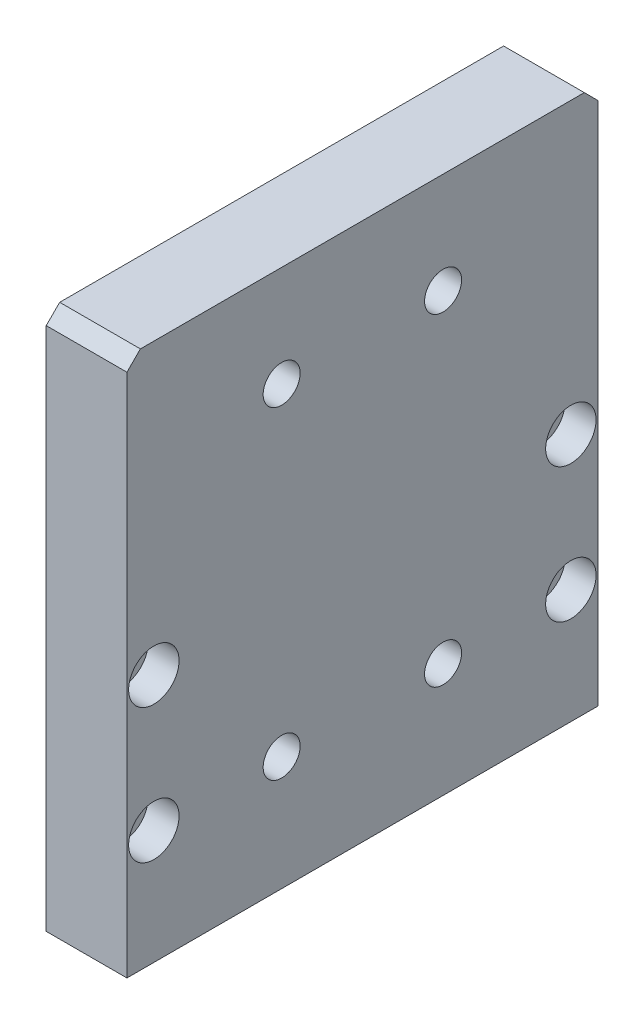
SolidWorks part; units mm, degrees
material "A6061"
ref_plane "前基準面" through (0, 0, 0) normal (0, 0, 1) x (1, 0, 0)
ref_plane "上基準面" through (0, 0, 0) normal (0, 1, 0) x (1, 0, 0)
ref_plane "右基準面" through (0, 0, 0) normal (1, 0, 0) x (0, 0, -1)
sketch "草图1" plane through (0, 0, 0) normal (1, 0, 0) x (0, 0, -1)
  line L1 (-35, 40) -> (35, 40)
  line L2 (-35, 40) -> (-35, -40)
  line L3 (-35, -40) -> (35, -40)
  line L4 (35, 40) -> (35, -40)
  line L5 (-35, 40) -> (35, -40) construction
  line L6 (-35, -40) -> (35, 40) construction
  point P0 (0, 0)
  dimension "D1" = 80
  dimension "D2" = 70
extrude "凸台-拉伸1" add sketch "草图1" along normal blind 12
hole_wizard "M5 六角圆柱头螺钉的柱形沉头孔1" positions "草图2" profile "草图3" counterbore size "M5" standard "GB" end condition through all
sketch "草图2" plane through (0, 0, 0) normal (-1, 0, 0) x (0, 0, 1)
  line L0 (0, 0) -> (0, -50.847) construction
  line L1 (-35, 40) -> (35, 40) construction
  point P0 (-12, 25)
  point P12 (-12, -23)
  point P14 (12, -23)
  point P15 (12, 25)
  dimension "D1" = 24
  dimension "D2" = 48
  dimension "D3" = 15
sketch "草图3" plane through (0, 25, -12) normal (0, 1, 0) x (0, 0, 1)
  line L0 (0, 0) -> (0, 12)
  line L1 (0, 12) -> (2.75, 12)
  line L3 (2.75, 12) -> (2.75, 5.7)
  line L4 (2.75, 5.7) -> (5, 5.7)
  line L5 (5, 5.7) -> (5, 0)
  line L7 (5, 0) -> (0, 0)
  line L11 (0, -6.35) -> (0, 107.95) construction
  dimension "通孔孔直径" = 5.5
  dimension "通孔孔深度" = 12
  dimension "柱形沉头孔直径" = 10
  dimension "柱形沉头孔深度" = 5.7
hole_wizard "M4 六角圆柱头螺钉的柱形沉头孔1" positions "草图4" profile "草图5" counterbore size "M4" standard "GB" end condition through all
sketch "草图4" plane through (12, 0, 0) normal (1, 0, 0) x (0, 0, -1)
  line L0 (0, 0) -> (0, -45.1266) construction
  line L2 (-35, -40) -> (35, -40) construction
  point P0 (-31, -23)
  point P3 (-31, -3)
  point P13 (31, -3)
  point P14 (31, -23)
  dimension "D1" = 62
  dimension "D2" = 20
  dimension "D3" = 17
sketch "草图5" plane through (12, -23, 31) normal (0, 1, 0) x (0, 0, -1)
  line L0 (0, 0) -> (0, 12)
  line L1 (0, 12) -> (2.25, 12)
  line L3 (2.25, 12) -> (2.25, 4.6)
  line L4 (2.25, 4.6) -> (3.75, 4.6)
  line L5 (3.75, 4.6) -> (3.75, 0)
  line L7 (3.75, 0) -> (0, 0)
  line L11 (0, -6.35) -> (0, 107.95) construction
  dimension "通孔孔直径" = 4.5
  dimension "通孔孔深度" = 12
  dimension "柱形沉头孔直径" = 7.5
  dimension "柱形沉头孔深度" = 4.6
sketch "草图6" plane through (0, -40, 0) normal (0, -1, 0) x (-1, 0, 0)
  line L0 (0, 0) -> (-12, 0) construction
  line L1 (-12, -35) -> (-12, 35) construction
  line L3 (-6, 0) -> (-6, 19.334) construction
  point P0 (-6, 22.5)
  point P9 (-6, -22.5)
  dimension "D1" = 45
hole_wizard "M4 螺纹孔1" positions "草图6" profile "草图7" tap size "M4" standard "GB"
sketch "草图7" plane through (6, -40, -22.5) normal (1, 0, 0) x (0, 0, -1)
  line L0 (0, 0) -> (0, 11.0914)
  line L1 (0, 11.0914) -> (1.65, 10.1)
  line L2 (1.65, 10.1) -> (1.65, 0)
  line L5 (1.65, 0) -> (0, 0)
  line L10 (0, 11.0914) -> (-1.65, 10.1) construction
  line L11 (0, -6.35) -> (0, 107.95) construction
  dimension "螺纹孔钻头直径" = 3.3
  dimension "螺纹孔钻头深度" = 10.1
  dimension "导头角度" = 118
cosmetic thread "孔螺纹线1" parameters "D1"=8, "D2"=4
cosmetic thread "孔螺纹线2" parameters "D1"=8, "D2"=4
chamfer "倒角1" distance 2 angle 45 2 edges at (6, 40, 35) (6, 40, -35)
